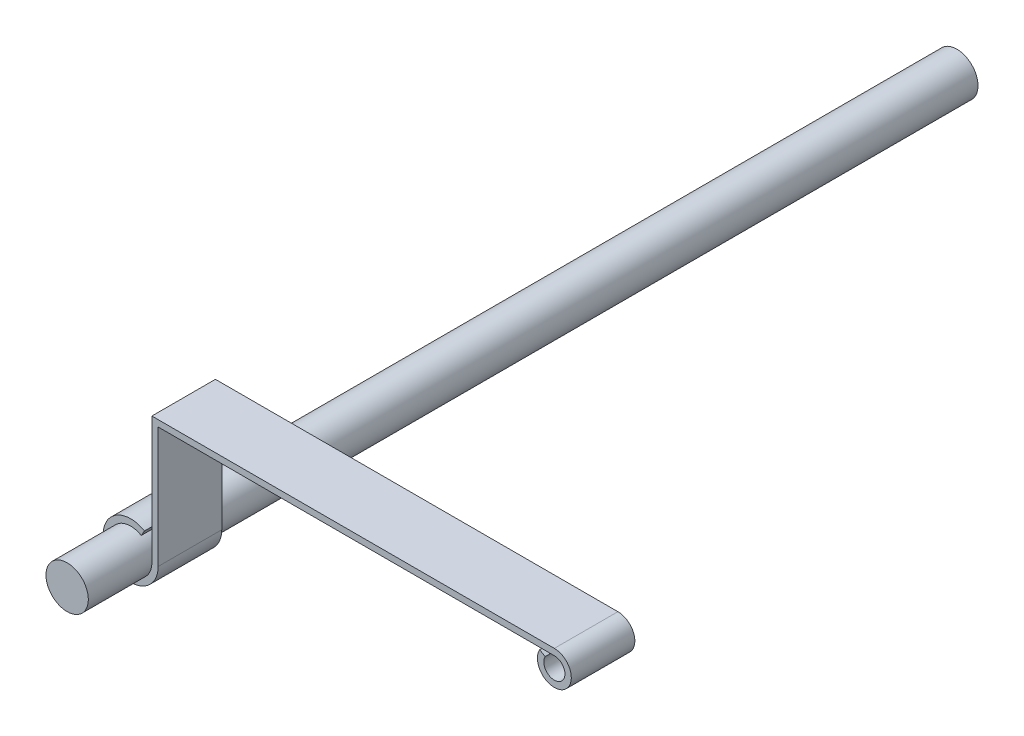
SolidWorks part; units mm, degrees
ref_plane "Front Plane" through (0, 0, 0) normal (0, 0, 1) x (1, 0, 0)
ref_plane "Top Plane" through (0, 0, 0) normal (0, 1, 0) x (1, 0, 0)
ref_plane "Right Plane" through (0, 0, 0) normal (1, 0, 0) x (0, 0, -1)
sketch "Sketch1" plane through (0, 0, 0) normal (0, 1, 0) x (1, 0, 0)
  line L0 (10, -15) -> (0, -15)
  line L1 (0, -15) -> (0, -45)
  line L2 (0, -45) -> (10, -45)
  line L3 (10, -45) -> (10, -15)
  line L4 (0, -15) -> (0, -45) construction
revolve "Revolve1" add sketch "Sketch1" angle 360 about L4
sketch "Sketch2" plane through (0, 0, 15) normal (0, 0, -1) x (-1, 0, 0)
  line L0 (-5, 8.6603) -> (-6.5, 11.2583)
  line L1 (-13, 0) -> (-13, 57)
  line L2 (-13, 57) -> (-200, 57)
  line L3 (-195.6699, 54.5) -> (-193.0718, 56)
  line L4 (-200, 60) -> (-10, 60)
  line L5 (-10, 60) -> (-10, 0)
  arc A0 (-6.5, 11.2583) -> (-13, 0) centre (0, 0) cw
  arc A1 (-200, 57) -> (-195.6699, 54.5) centre (-200, 52) ccw
  arc A2 (-193.0718, 56) -> (-200, 60) centre (-200, 52) cw
  arc A3 (-10, 0) -> (-5, 8.6603) centre (0, 0) cw
extrude "Boss-Extrude1" add sketch "Sketch2" along normal blind 30
sketch "Sketch3" plane through (0, 0, -15) normal (0, 0, -1) x (-1, 0, 0)
  circle A0 centre (0, 0) radius 10
extrude "Boss-Extrude2" add sketch "Sketch3" along normal blind 360
